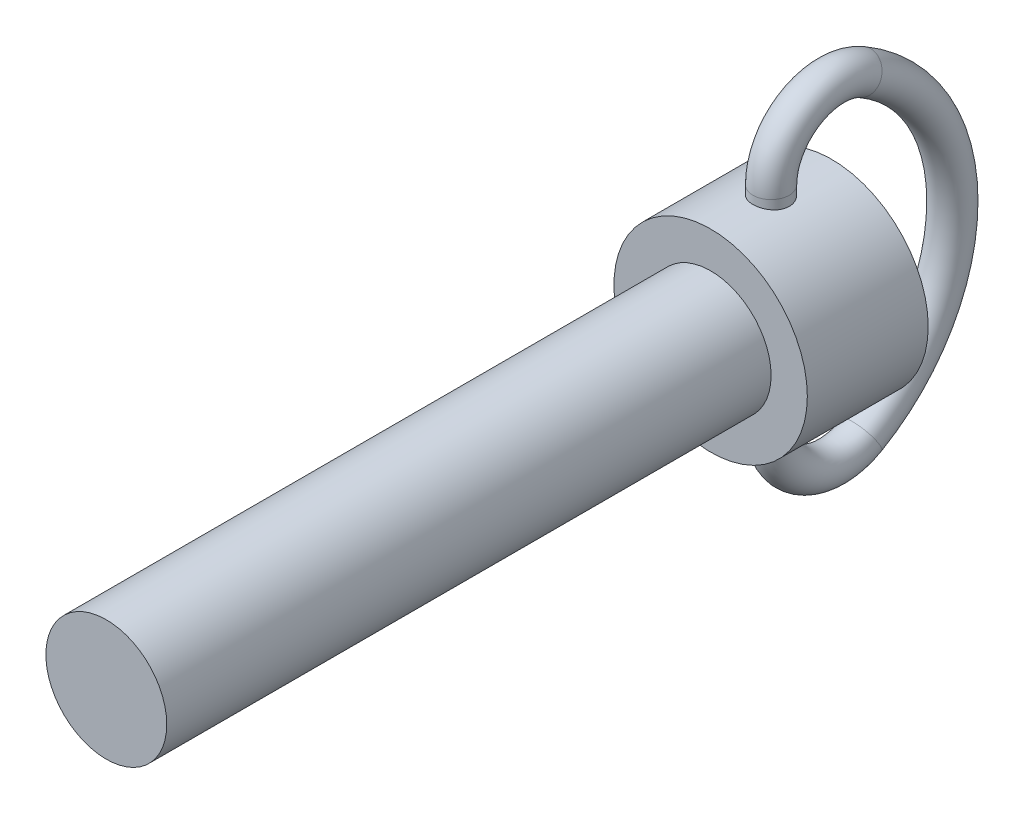
from build123d import *

# Parameters (mm, degrees)
SKETCH1_R           = 4
BOSS_EXTRUDE1_DEPTH = 5
SKETCH2_R           = 2.5
BOSS_EXTRUDE2_DEPTH = 25
SKETCH3_R           = 0.75


with BuildPart() as part:
    # Sketch1 → Boss-Extrude1 (new body)
    with BuildSketch(Plane.XY):
        Circle(SKETCH1_R)
    extrude(amount=BOSS_EXTRUDE1_DEPTH)

    # Sketch2 → Boss-Extrude2 (add)
    with BuildSketch(Plane.XY.offset(5)):
        Circle(SKETCH2_R)
    extrude(amount=BOSS_EXTRUDE2_DEPTH)

    # Sweep1: sweep along a path in Sketch4
    with BuildLine(Plane(origin=(0, 0, 0), x_dir=(0, 0, -1), z_dir=(1, 0, 0))) as sweep1_path:
        Line((-2.5, 0), (-2.5, -4.330127019))
        ThreePointArc((-2.5, -4.330127019), (-1.25, -6.495190528), (1.25, -6.495190528))
        ThreePointArc((1.25, -6.495190528), (5, 0), (1.25, 6.495190528))
        ThreePointArc((1.25, 6.495190528), (-1.25, 6.495190528), (-2.5, 4.330127019))
        Line((-2.5, 4.330127019), (-2.5, 0))
    # Sketch3 → Sweep1 (sweep)
    with BuildSketch(Plane(origin=(0, 0, 0), x_dir=(1, 0, 0), z_dir=(0, 1, 0))):
        with Locations((0, -2.5)):
            Circle(SKETCH3_R)
    sweep(path=sweep1_path.line)


solid = part.part
